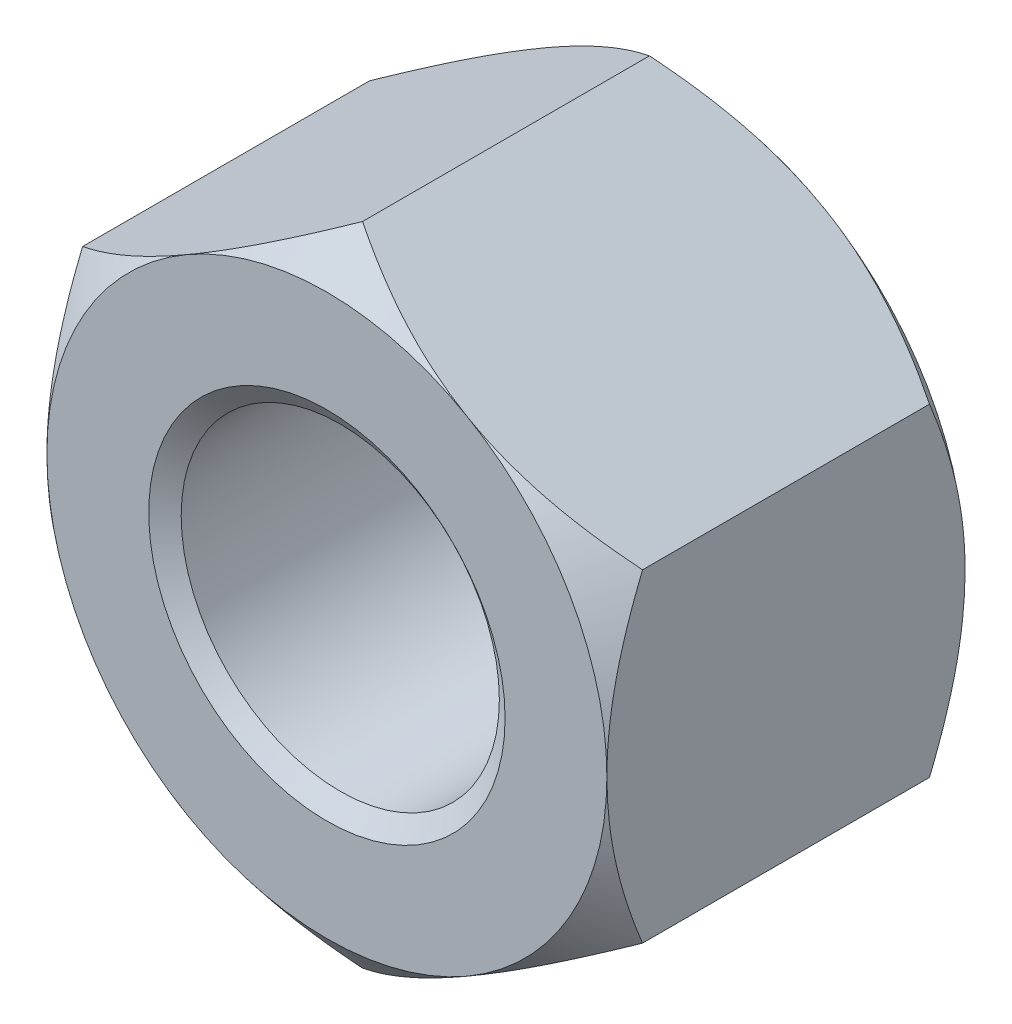
from build123d import *

# Parameters (mm, degrees)
BASENUT_START = -44.6786
BASENUTSKE_R  = 19.84375
BASENUT_DEPTH = 44.6786


with BuildPart() as part:
    # BaseNutSke → BaseNut (new body)
    with BuildSketch(Plane.XY.offset(BASENUT_START)):
        Polygon((34.925, 20.163958151), (34.925, -20.163958151), (0, -40.327916303), (-34.925, -20.163958151), (-34.925, 20.163958151), (0, 40.327916303), align=None)
        Circle(BASENUTSKE_R, mode=Mode.SUBTRACT)
    extrude(amount=BASENUT_DEPTH)

    # Sketch3 → Double-Chamfer (revolve, cut)
    with BuildSketch(Plane(origin=(0, 0, 0), x_dir=(0, 0, -1), z_dir=(1, 0, 0))):
        Polygon((44.6786, 34.925), (40.2336, 40.327916303), (40.2336, 53.027916303), (57.3786, 53.027916303), (57.3786, 34.925), align=None)
        Polygon((4.445, 53.027916303), (-12.7, 53.027916303), (-12.7, 34.925), (0, 34.925), (4.445, 40.327916303), align=None)
    revolve(axis=Axis((0, 0, 0), (0, 0, -1)), mode=Mode.SUBTRACT)

    # Sketch5 → EndChamfer (revolve, cut)
    with BuildSketch(Plane(origin=(0, 0, 0), x_dir=(0, 0, -1), z_dir=(1, 0, 0)), mode=Mode.PRIVATE) as endchamfer_sk:
        Polygon((44.6532, 22.225), (42.81909388, 19.605625), (44.704, 19.605625), (44.704, 22.225), align=None)
        Polygon((-0.0508, 22.225), (0, 22.225), (1.83410612, 19.605625), (-0.0508, 19.605625), align=None)
    revolve(endchamfer_sk.sketch.rotate(Axis((0, 0, -25.037505729), (0, 0, -1)), 90), axis=Axis((0, 0, -25.037505729), (0, 0, -1)), mode=Mode.SUBTRACT)


solid = part.part
